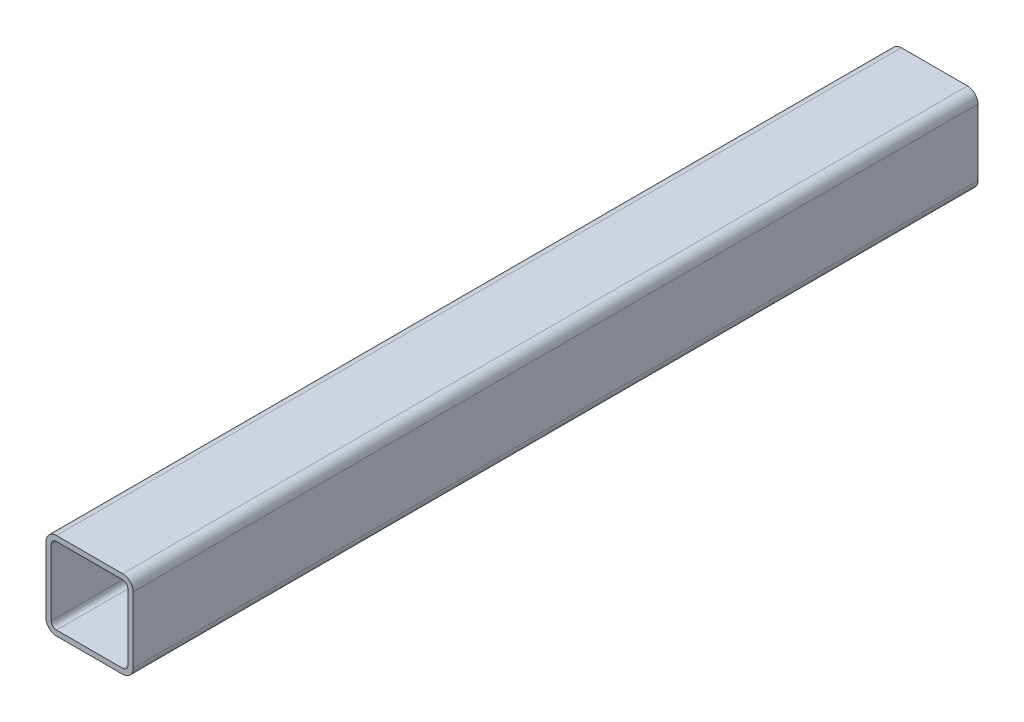
from build123d import *

# Parameters (mm, degrees)
GB_6728_1986_050_X_50_X_3_1_DEPTH = 485


with BuildPart() as part:
    # Sketch1 → Gb／6728-1986方形空心型钢 050 X 50 X 3(1) (new body)
    with BuildSketch(Plane.YX.offset(-242.5)):
        with BuildLine():
            Line((-19, -25), (19, -25))
            ThreePointArc((19, -25), (23.242640687, -23.242640687), (25, -19))
            Line((25, -19), (25, 19))
            ThreePointArc((25, 19), (23.242640687, 23.242640687), (19, 25))
            Line((19, 25), (-19, 25))
            ThreePointArc((-19, 25), (-23.242640687, 23.242640687), (-25, 19))
            Line((-25, 19), (-25, -19))
            ThreePointArc((-25, -19), (-23.242640687, -23.242640687), (-19, -25))
        make_face()
        with BuildLine():
            Line((-19, -22), (19, -22))
            ThreePointArc((19, -22), (21.121320344, -21.121320344), (22, -19))
            Line((22, -19), (22, 19))
            ThreePointArc((22, 19), (21.121320344, 21.121320344), (19, 22))
            Line((19, 22), (-19, 22))
            ThreePointArc((-19, 22), (-21.121320344, 21.121320344), (-22, 19))
            Line((-22, 19), (-22, -19))
            ThreePointArc((-22, -19), (-21.121320344, -21.121320344), (-19, -22))
        make_face(mode=Mode.SUBTRACT)
    extrude(amount=GB_6728_1986_050_X_50_X_3_1_DEPTH)


solid = part.part
